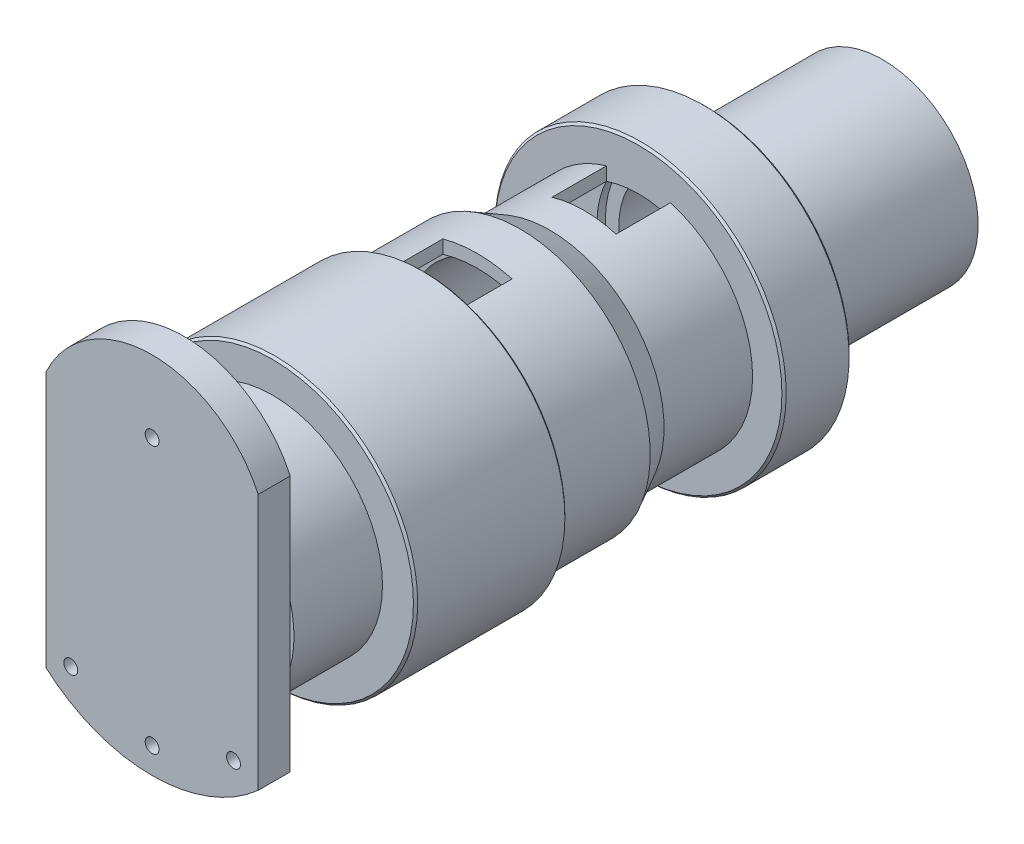
from build123d import *

# Parameters (mm, degrees)
EXTRUDE_1_DEPTH     = 30
SKETCH_3_R          = 103
SKETCH_3_R_2        = 93
EXTRUDE_2_DEPTH     = 85
CHAMFER_1_SIZE      = 2
CHAMFER_1_SIZE2     = 2.444922552
CHAMFER_2_SIZE      = 2
SKETCH_5_W          = 50
SKETCH_5_H          = 65
SKETCH_5_W_2        = 51
SKETCH_5_H_2        = 60
CUT_EXTRUDE_1_DEPTH = 145
CUT_EXTRUDE_2_REACH = 738.023
SKETCH_6_R          = 6.5
SKETCH_7_W          = 8
SKETCH_7_H          = 290.552201754
SKETCH_7_H_2        = 289.758517494
CUT_EXTRUDE_3_DEPTH = 30


with BuildPart() as part:
    # 草图2 → 凸台-拉伸1 (new body)
    with BuildSketch(Plane.XY):
        with BuildLine():
            Line((-107.5, 21.352049082), (-107.5, -186.717950918))
            ThreePointArc((-107.5, -186.717950918), (0, -232.105571153), (107.5, -186.717950918))
            Line((107.5, -186.717950918), (107.5, 21.352049082))
            ThreePointArc((107.5, 21.352049082), (0, 109.6), (-107.5, 21.352049082))
        make_face()
    extrude(amount=EXTRUDE_1_DEPTH)

    # 草图3 → 凸台-拉伸2 (add)
    with BuildSketch(Plane(origin=(0, 0, 0), x_dir=(-1, 0, 0), z_dir=(0, 0, -1))):
        with Locations(Location((0, -82.682950918, 0), (0, 0, 180))):
            Circle(SKETCH_3_R)
        with Locations((0, -82.682950918)):
            Circle(SKETCH_3_R_2, mode=Mode.SUBTRACT)
    extrude(amount=EXTRUDE_2_DEPTH)

    # 草图4 → 旋转1 (revolve)
    with BuildSketch(Plane.ZX.offset(-82.682950918)):
        Polygon((-95, -93), (-95, -122), (-213, -122), (-213, -110), (-303, -110), (-303, -95), (-438, -95), (-438, -124.5), (-477, -124.5), (-477, -90), (-485, -90), (-485, -77.5), (-655, -77.5), (-655, -89.5), (-497, -89.5), (-489, -136.5), (-426, -136.5), (-426, -107), (-343, -107), (-315, -122), (-225, -122), (-225, -134), (-83, -134), (-83, -93), align=None)
    revolve(axis=Axis((0, -82.682950918, -1172.450178842), (0, 0, 1)))

    # 倒角1
    chamfer_1_edges = [part.edges().sort_by_distance(p)[0] for p in [
        (136.5, -82.682950918, -489),
    ]]
    chamfer_1_side = [part.faces().sort_by_distance(p)[0] for p in [
        (136.5, -82.682950918, -457.5),
    ]]
    chamfer(chamfer_1_edges, length=CHAMFER_1_SIZE, length2=CHAMFER_1_SIZE2, reference=chamfer_1_side[0])

    # 倒角2
    chamfer_2_edges = [part.edges().sort_by_distance(p)[0] for p in [
        (134, -82.682950918, -83),
        (134, -82.682950918, -225),
        (136.5, -82.682950918, -426),
    ]]
    chamfer(chamfer_2_edges, length=CHAMFER_2_SIZE)

    # 草图5 → 切除-拉伸1 (cut)
    with BuildSketch(Plane.ZX.offset(-82.682950918)):
        with Locations((-250, 0)):
            Rectangle(SKETCH_5_W, SKETCH_5_H)
        with Locations((-400.5, 0)):
            Rectangle(SKETCH_5_W_2, SKETCH_5_H_2)
    extrude(amount=CUT_EXTRUDE_1_DEPTH, mode=Mode.SUBTRACT)

    # 草图6 → 切除-拉伸2 (cut, up to next)
    with BuildSketch(Plane.XY.offset(30), mode=Mode.PRIVATE) as cut_extrude_2_sk1:
        with Locations((0, 42.317049082)):
            Circle(SKETCH_6_R)
    cut_extrude_2_tool1 = extrude(cut_extrude_2_sk1.sketch, amount=-CUT_EXTRUDE_2_REACH, mode=Mode.PRIVATE) & part.part
    # 草图6 → 切除-拉伸2 (cut, up to next)
    with BuildSketch(Plane.XY.offset(30), mode=Mode.PRIVATE) as cut_extrude_2_sk2:
        with Locations((0, -207.682950918)):
            Circle(SKETCH_6_R)
    cut_extrude_2_tool2 = extrude(cut_extrude_2_sk2.sketch, amount=-CUT_EXTRUDE_2_REACH, mode=Mode.PRIVATE) & part.part
    # 草图6 → 切除-拉伸2 (cut, up to next)
    with BuildSketch(Plane.XY.offset(30), mode=Mode.PRIVATE) as cut_extrude_2_sk3:
        with Locations((-76.315136113, -181.682950918)):
            Circle(SKETCH_6_R)
    cut_extrude_2_tool3 = extrude(cut_extrude_2_sk3.sketch, amount=-CUT_EXTRUDE_2_REACH, mode=Mode.PRIVATE) & part.part
    # 草图6 → 切除-拉伸2 (cut, up to next)
    with BuildSketch(Plane.XY.offset(30), mode=Mode.PRIVATE) as cut_extrude_2_sk4:
        with Locations((76.315136113, -181.682950918)):
            Circle(SKETCH_6_R)
    cut_extrude_2_tool4 = extrude(cut_extrude_2_sk4.sketch, amount=-CUT_EXTRUDE_2_REACH, mode=Mode.PRIVATE) & part.part
    add(cut_extrude_2_tool1.solids().sort_by_distance((0, 42.317049, 30))[0], mode=Mode.SUBTRACT)
    add(cut_extrude_2_tool2.solids().sort_by_distance((0, -207.682951, 30))[0], mode=Mode.SUBTRACT)
    add(cut_extrude_2_tool3.solids().sort_by_distance((-76.315136, -181.682951, 30))[0], mode=Mode.SUBTRACT)
    add(cut_extrude_2_tool4.solids().sort_by_distance((76.315136, -181.682951, 30))[0], mode=Mode.SUBTRACT)

    # 草图7 → 切除-拉伸3 (cut)
    with BuildSketch(Plane.XY.offset(30)):
        with Locations((-103.5, -82.682950918)):
            Rectangle(SKETCH_7_W, SKETCH_7_H)
        with Locations((103.5, -82.682950918)):
            Rectangle(SKETCH_7_W, SKETCH_7_H_2)
    extrude(amount=-CUT_EXTRUDE_3_DEPTH, mode=Mode.SUBTRACT)


solid = part.part
